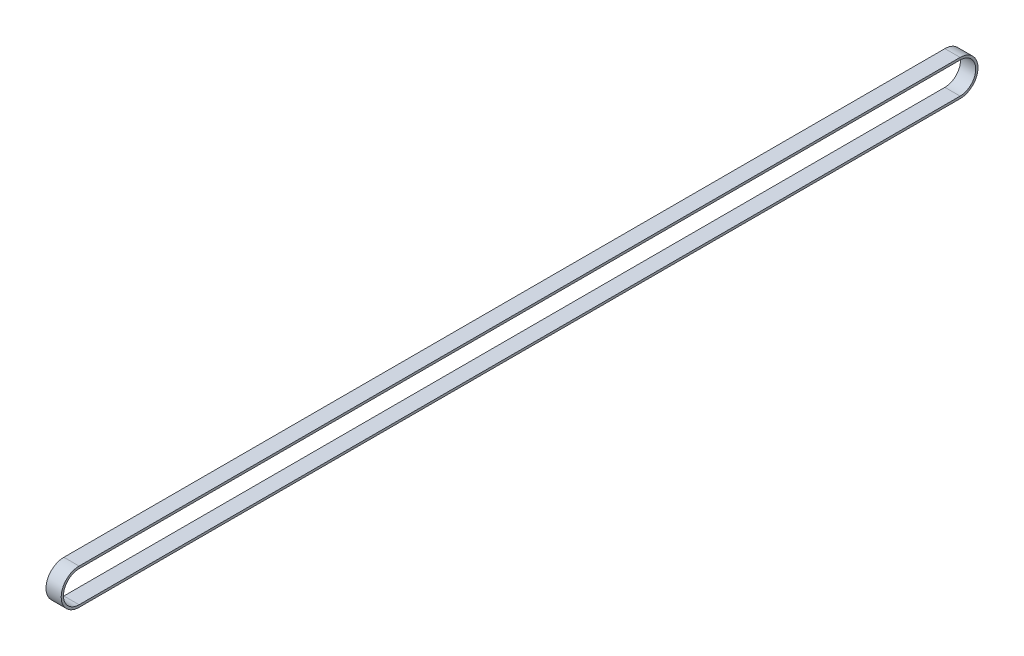
SolidWorks part; units mm, degrees
material "聚脂树脂"
ref_plane "前视基准面" through (0, 0, 0) normal (0, 0, 1) x (1, 0, 0)
ref_plane "上视基准面" through (0, 0, 0) normal (0, 1, 0) x (1, 0, 0)
ref_plane "右视基准面" through (0, 0, 0) normal (1, 0, 0) x (0, 0, -1)
sketch "草图2" plane through (0, 0, 0) normal (1, 0, 0) x (0, 0, -1)
  line L0 (0, 31.85) -> (-1740, 31.85)
  line L6 (-1740, -31.85) -> (0, -31.85)
  arc A0 (0, -31.85) -> (0, 31.85) centre (0, 0) ccw
  arc A1 (-1740, 31.85) -> (-1740, -31.85) centre (-1740, 0) ccw
  dimension "D2" = 63.7
  dimension "D7" = 1740
extrude "拉伸-薄壁1" add sketch "草图2" along normal mid plane 30 thin
